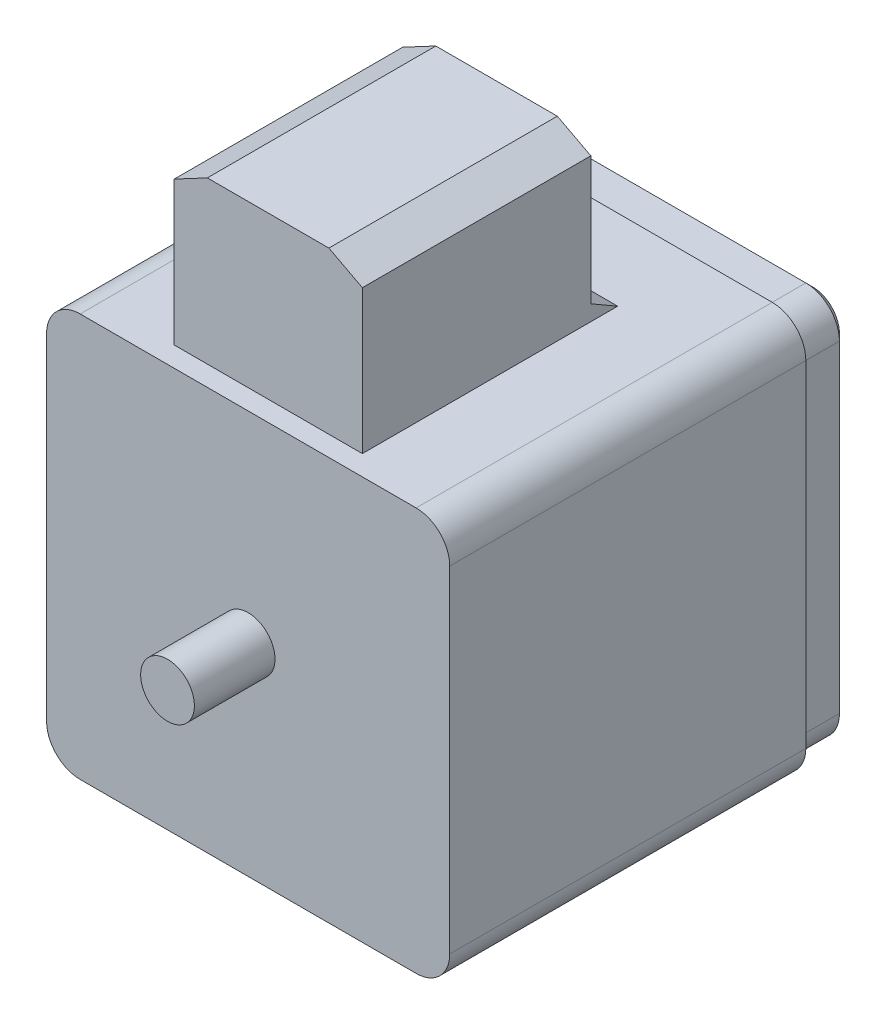
SolidWorks part; units mm, degrees
ref_plane "前视基准面" through (0, 0, 0) normal (0, 0, 1) x (1, 0, 0)
ref_plane "上视基准面" through (0, 0, 0) normal (0, 1, 0) x (1, 0, 0)
ref_plane "右视基准面" through (0, 0, 0) normal (1, 0, 0) x (0, 0, -1)
sketch "草图1" plane through (0, 0, 0) normal (0, 0, 1) x (1, 0, 0)
  line L1 (-30, -30) -> (30, -30)
  line L2 (-30, -30) -> (-30, 30)
  line L3 (-30, 30) -> (30, 30)
  line L4 (30, -30) -> (30, 30)
  line L5 (-30, -30) -> (30, 30) construction
  line L6 (-30, 30) -> (30, -30) construction
  point P0 (0, 0)
  dimension "D1" = 60
  dimension "D2" = 60
extrude "凸台-拉伸1" add sketch "草图1" along normal blind 60
sketch "草图2" plane through (0, 0, 60) normal (0, 0, 1) x (1, 0, 0)
  circle A0 centre (0, 0) radius 4
  dimension "D1" = 8
extrude "凸台-拉伸2" add sketch "草图2" along normal blind 12
sketch "草图3" plane through (0, 0, 0) normal (0, 0, -1) x (-1, 0, 0)
  line L1 (-30, -30) -> (30, -30)
  line L2 (-30, -30) -> (-30, 30)
  line L3 (-30, 30) -> (30, 30)
  line L4 (30, -30) -> (30, 30)
  line L5 (-30, -30) -> (30, 30) construction
  line L6 (-30, 30) -> (30, -30) construction
  line L7 (-29, -29) -> (29, -29)
  line L8 (-29, -29) -> (-29, 29)
  line L9 (-29, 29) -> (29, 29)
  line L10 (29, -29) -> (29, 29)
  line L11 (-29, -29) -> (29, 29) construction
  line L12 (-29, 29) -> (29, -29) construction
  point P0 (0, 0)
  point P7 (0, 0)
  dimension "D1" = 1
extrude "切除-拉伸1" cut sketch "草图3" against normal blind 7
fillet "圆角1" radius 5 4 edges at (-29, 29, 3.5) (-29, -29, 3.5) (29, -29, 3.5) (29, 29, 3.5)
chamfer "倒角1" distance 1 angle 45 8 edges at (-27.5355, 27.5355, 0) (-29, 0, 0) (-27.5355, -27.5355, 0) (0, -29, 0) (27.5355, -27.5355, 0) (29, 0, 0) (27.5355, 27.5355, 0) (0, 29, 0)
sketch "草图4" plane through (0, 0, 60) normal (0, 0, 1) x (1, 0, 0)
  line L0 (30, 30) -> (-30, 30) construction
  line L1 (-30, -30) -> (30, -30)
  line L2 (-30, -30) -> (-30, 30)
  line L3 (-30, 30) -> (30, 30)
  line L4 (30, -30) -> (30, 30)
  line L5 (-30, -30) -> (30, 30) construction
  line L6 (-30, 30) -> (30, -30) construction
  point P0 (0, 0)
fillet "圆角2" radius 5 4 edges at (30, 30, 33.5) (30, -30, 33.5) (-30, -30, 33.5) (-30, 30, 33.5)
ref_plane "基准面1" through (0, 30, 0) normal (0, 1, 0) x (1, 0, 0)
sketch "草图5" plane through (0, 30, 0) normal (0, 1, 0) x (1, 0, 0)
  line L1 (-14, -57) -> (14, -57)
  line L2 (14, -57) -> (14, -19)
  line L3 (14, -19) -> (-14, -19)
  line L4 (-30, -60) -> (30, -60) construction
  line L5 (-14, -57) -> (-14, -19)
  dimension "D1" = 3
  dimension "D2" = 38
  dimension "D3" = 28
extrude "凸台-拉伸3" add sketch "草图5" along normal blind 24
sketch "草图6" plane through (0, 0, 19) normal (0, 0, -1) x (-1, 0, 0)
  line L1 (-22.5921, 59.89) -> (21.636, 59.89)
  line L2 (-22.5921, 59.89) -> (-22.5921, 30)
  line L3 (-22.5921, 30) -> (21.636, 30)
  line L4 (21.636, 59.89) -> (21.636, 30)
  line L6 (-14, 30) -> (14, 30) construction
  circle A0 centre (0, 42) radius 7.0836
  dimension "D1" = 0
extrude "切除-拉伸2" cut sketch "草图6" against normal blind 4 draft 30
sketch "草图7" plane through (0, 0, 23) normal (0, 0, -1) x (-1, 0, 0)
  line L0 (-14, 51.3832) -> (-9.0157, 54)
  line L1 (-14, 54) -> (-14, 32.3094) construction
  line L2 (-14, 54) -> (14, 54) construction
  line L3 (-9.0157, 54) -> (9.0734, 54)
  line L4 (9.0734, 54) -> (14, 51.3832)
  line L5 (14, 32.3094) -> (14, 54) construction
  line L6 (14, 51.3832) -> (16.4921, 52.6916)
  line L7 (16.4921, 52.6916) -> (15.2461, 56.5515)
  line L8 (15.2461, 56.5515) -> (-18.0041, 56.5515)
  line L9 (-18.0041, 56.5515) -> (-14, 51.3832)
extrude "切除-拉伸3" cut sketch "草图7" against normal through all
